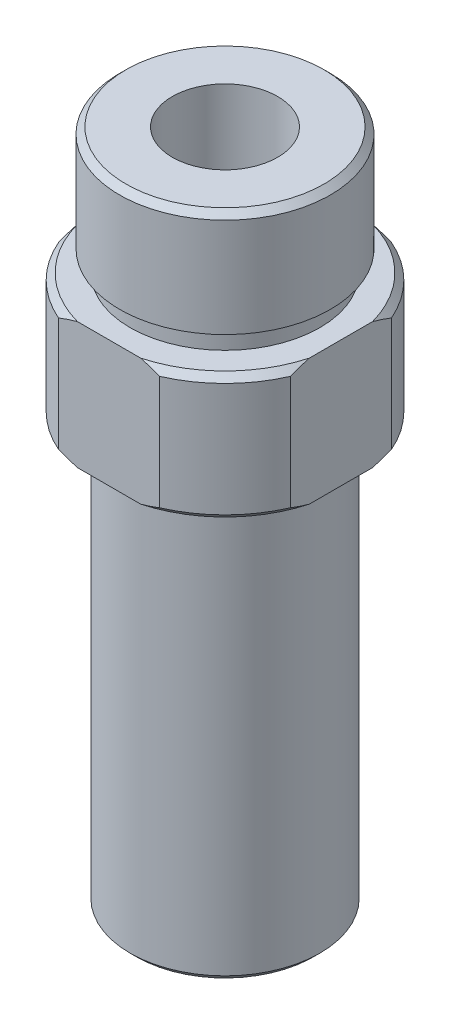
from build123d import *

# Parameters (mm, degrees)
SKETCH_1_R            = 5
EXTRUDE_1_DEPTH       = 6
SKETCH_2_R            = 6
EXTRUDE_2_DEPTH       = 6
SKETCH_3_R            = 4.5
EXTRUDE_3_DEPTH       = 20
CHAMFER_1_SIZE        = 0.3
SKETCH_7_W            = 8.670570122
SKETCH_7_H            = 17.253558728
SKETCH_7_W_2          = 11.735923196
CUT_EXTRUDE_1_DEPTH   = 10
HOLE_WIZARD_5_0_5_1_D = 5
SKETCH_8_W            = 3.075789072
SKETCH_8_H            = 1
SKETCH_9_W            = 7.38579235
SKETCH_9_H            = 17.49729378
SKETCH_9_W_2          = 12.485506115
SKETCH_9_H_2          = 24.97101223
CUT_EXTRUDE_2_DEPTH   = 10
CHAMFER_7_SIZE        = 0.3


with BuildPart() as part:
    # 草图1 → 凸台-拉伸1 (new body)
    with BuildSketch(Plane(origin=(0, 0, 0), x_dir=(1, 0, 0), z_dir=(0, 1, 0))):
        with Locations(Location((0, 0, 0), (0, 0, 270))):
            Circle(SKETCH_1_R)
    extrude(amount=-EXTRUDE_1_DEPTH)

    # 草图2 → 凸台-拉伸2 (add)
    with BuildSketch(Plane.XZ.offset(6)):
        with Locations(Location((0, 0, 0), (0, 0, 270))):
            Circle(SKETCH_2_R)
    extrude(amount=EXTRUDE_2_DEPTH)

    # 草图3 → 凸台-拉伸3 (add)
    with BuildSketch(Plane.XZ.offset(12)):
        with Locations(Location((0, 0, 0), (0, 0, 270))):
            Circle(SKETCH_3_R)
    extrude(amount=EXTRUDE_3_DEPTH)

    # 倒角1
    chamfer_1_edges = [part.edges().sort_by_distance(p)[0] for p in [
        (0, 0, -5),
        (0, -6, 6),
        (0, -12, 6),
    ]]
    chamfer(chamfer_1_edges, length=CHAMFER_1_SIZE)

    # 草图7 → 切除-拉伸1 (cut, symmetric)
    with BuildSketch(Plane.XY):
        with Locations((-9.835285061, -4.858845759)):
            Rectangle(SKETCH_7_W, SKETCH_7_H)
        with Locations((11.367961598, -4.858845759)):
            Rectangle(SKETCH_7_W_2, SKETCH_7_H)
    extrude(amount=CUT_EXTRUDE_1_DEPTH, both=True, mode=Mode.SUBTRACT)

    # Ø5.0 (5) 直径孔1 (through all)
    with Locations(Plane(origin=(0, 0, 0), x_dir=(1, 0, 0), z_dir=(0, 1, 0))):
        with Locations((0, 0)):
            Hole(HOLE_WIZARD_5_0_5_1_D / 2)

    # 草图8 → 切除-旋转1 (revolve, cut)
    with BuildSketch(Plane.XY, mode=Mode.PRIVATE) as cut_revolve_1_sk:
        with Locations((-6.037894536, -5.5)):
            Rectangle(SKETCH_8_W, SKETCH_8_H)
    revolve(cut_revolve_1_sk.sketch.rotate(Axis((0, -6, 0), (0, 1, 0)), 270), axis=Axis((0, -6, 0), (0, 1, 0)), mode=Mode.SUBTRACT)

    # 草图9 → 切除-拉伸2 (cut, symmetric)
    with BuildSketch(Plane(origin=(0, 0, 0), x_dir=(0, 0, -1), z_dir=(1, 0, 0))):
        with Locations((-9.192896175, -6.091907364)):
            Rectangle(SKETCH_9_W, SKETCH_9_H)
        with Locations((11.742753057, -3.629976581)):
            Rectangle(SKETCH_9_W_2, SKETCH_9_H_2)
    extrude(amount=CUT_EXTRUDE_2_DEPTH, both=True, mode=Mode.SUBTRACT)

    # 倒角7
    chamfer_7_edges = [part.edges().sort_by_distance(p)[0] for p in [
        (0, -32, 4.5),
    ]]
    chamfer(chamfer_7_edges, length=CHAMFER_7_SIZE)


solid = part.part
